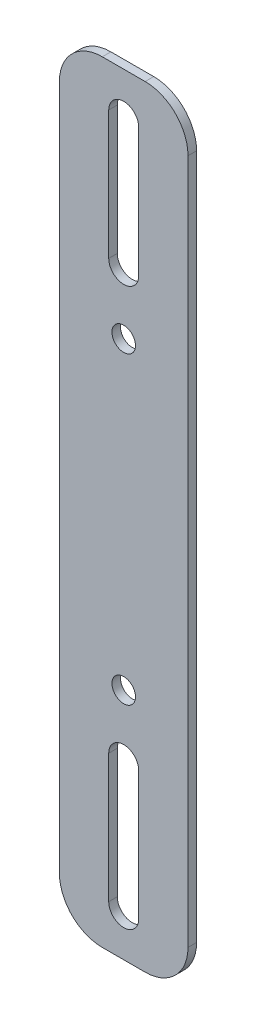
from build123d import *

# Parameters (mm, degrees)
SKETCH1_W           = 30
SKETCH1_H           = 180
BOSS_EXTRUDE1_DEPTH = 2
FILLET1_R           = 10
CUT_EXTRUDE1_DEPTH  = 92.263355187
SKETCH3_R           = 2.75
CUT_EXTRUDE2_DEPTH  = 92.263355187


with BuildPart() as part:
    # Sketch1 → Boss-Extrude1 (new body)
    with BuildSketch(Plane.XY):
        Rectangle(SKETCH1_W, SKETCH1_H)
    extrude(amount=BOSS_EXTRUDE1_DEPTH)

    # Fillet1
    fillet1_edges = [part.edges().sort_by_distance(p)[0] for p in [
        (-15, 90, 1),
        (15, 90, 1),
        (15, -90, 1),
        (-15, -90, 1),
    ]]
    fillet(fillet1_edges, radius=FILLET1_R)

    # Sketch2 → Cut-Extrude1 (cut, through all)
    with BuildSketch(Plane.XY.offset(2)):
        with BuildLine():
            Line((3.5, 80), (3.5, 50))
            ThreePointArc((3.5, 50), (0, 46.5), (-3.5, 50))
            Line((-3.5, 50), (-3.5, 80))
            ThreePointArc((-3.5, 80), (0, 83.5), (3.5, 80))
        make_face()
    cut_extrude1 = extrude(amount=-CUT_EXTRUDE1_DEPTH, mode=Mode.SUBTRACT)

    # Mirror1: Cut-Extrude1 across plane
    add(cut_extrude1.mirror(Plane.ZX), mode=Mode.SUBTRACT)

    # Sketch3 → Cut-Extrude2 (cut, through all)
    with BuildSketch(Plane.XY.offset(2)):
        with Locations((0, -35.5)):
            Circle(SKETCH3_R)
        with Locations((0, 35.5)):
            Circle(SKETCH3_R)
    extrude(amount=-CUT_EXTRUDE2_DEPTH, mode=Mode.SUBTRACT)


solid = part.part
